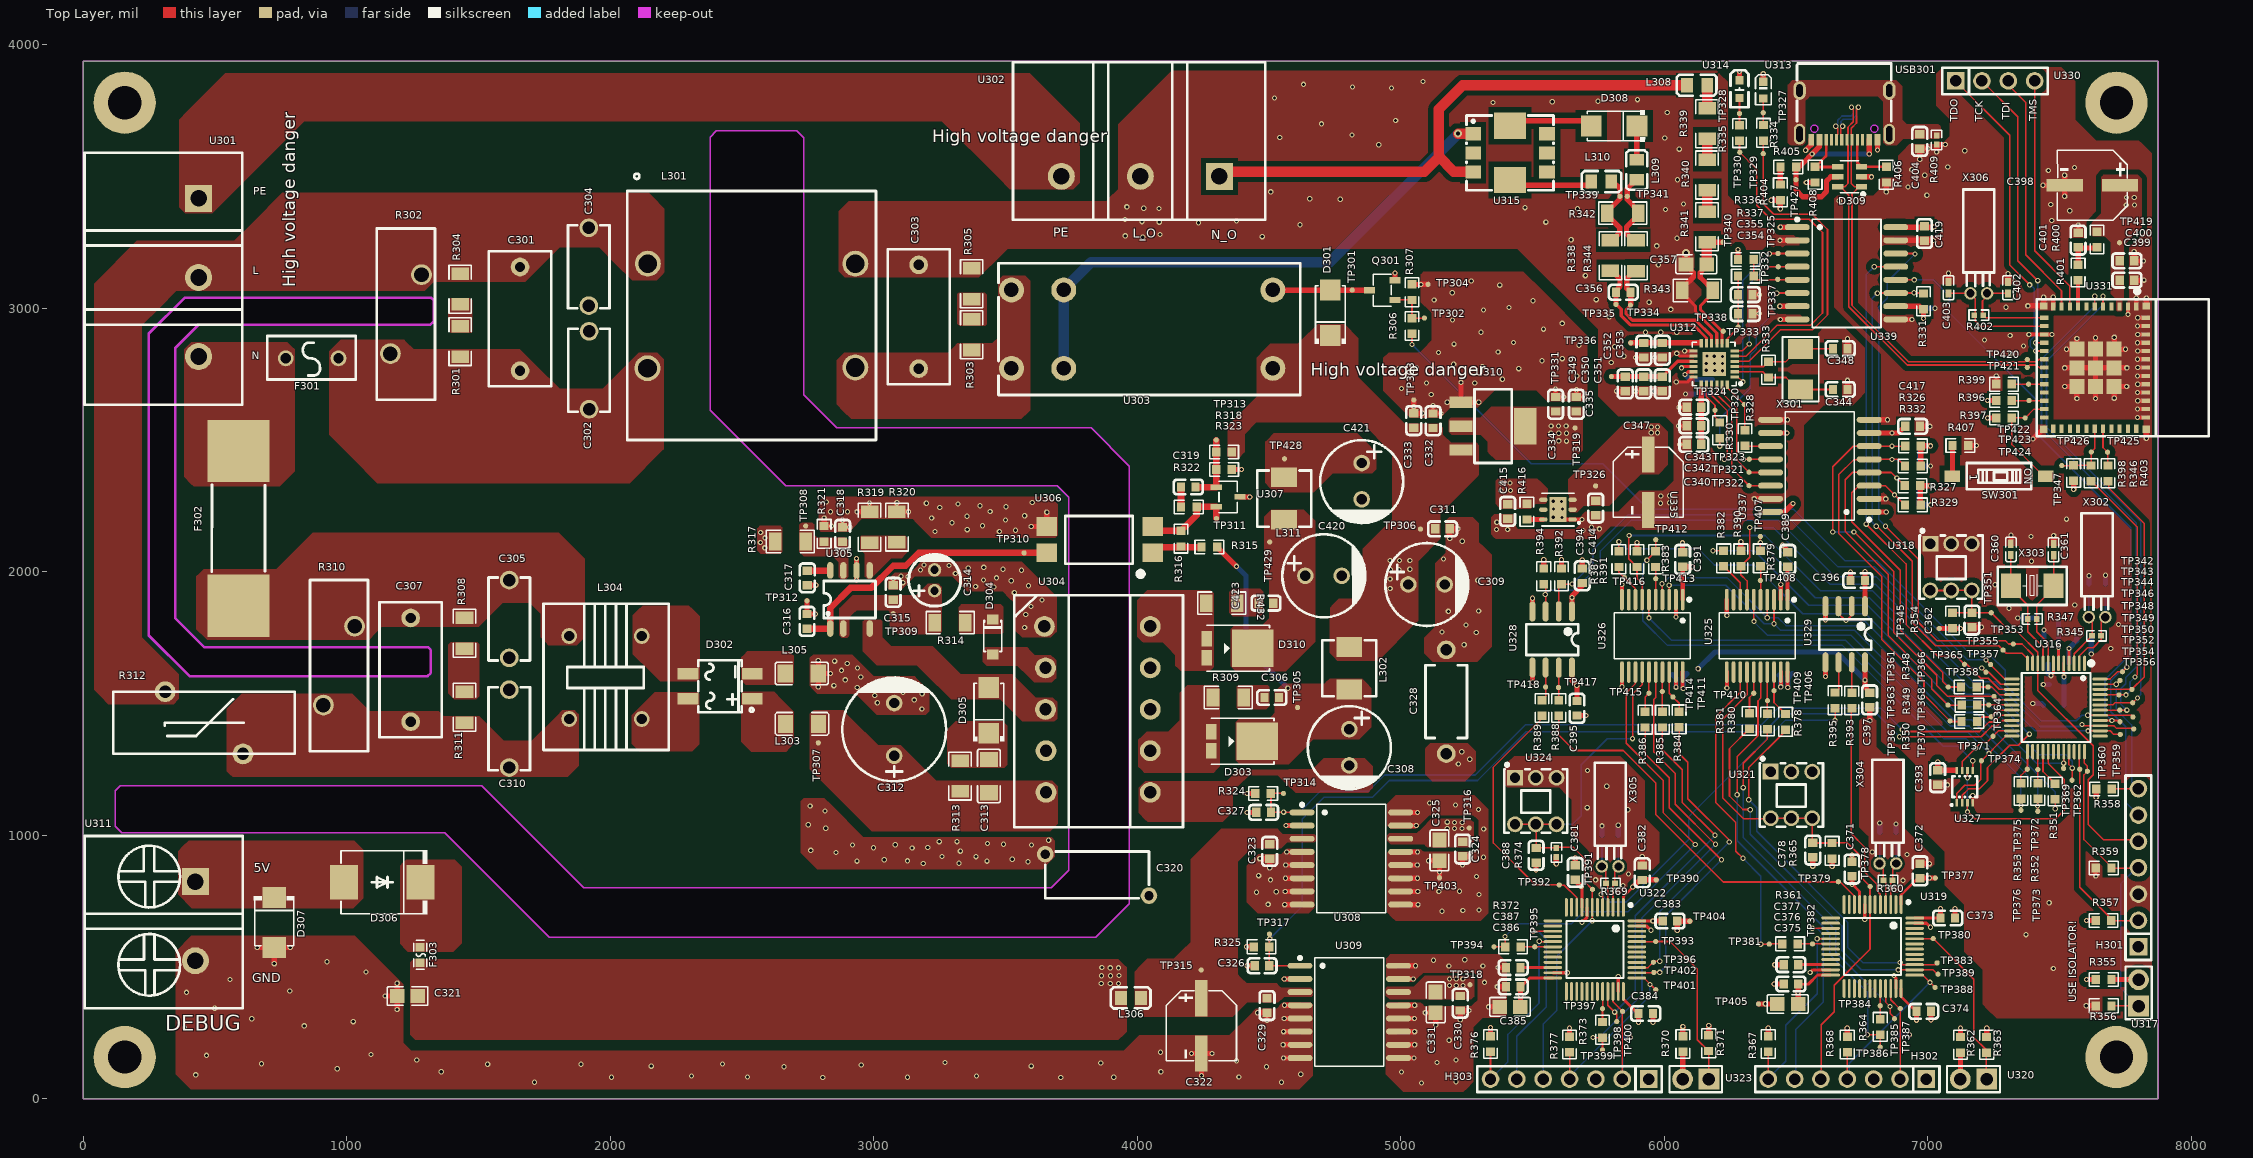
[diagram p0: Top Layer view]
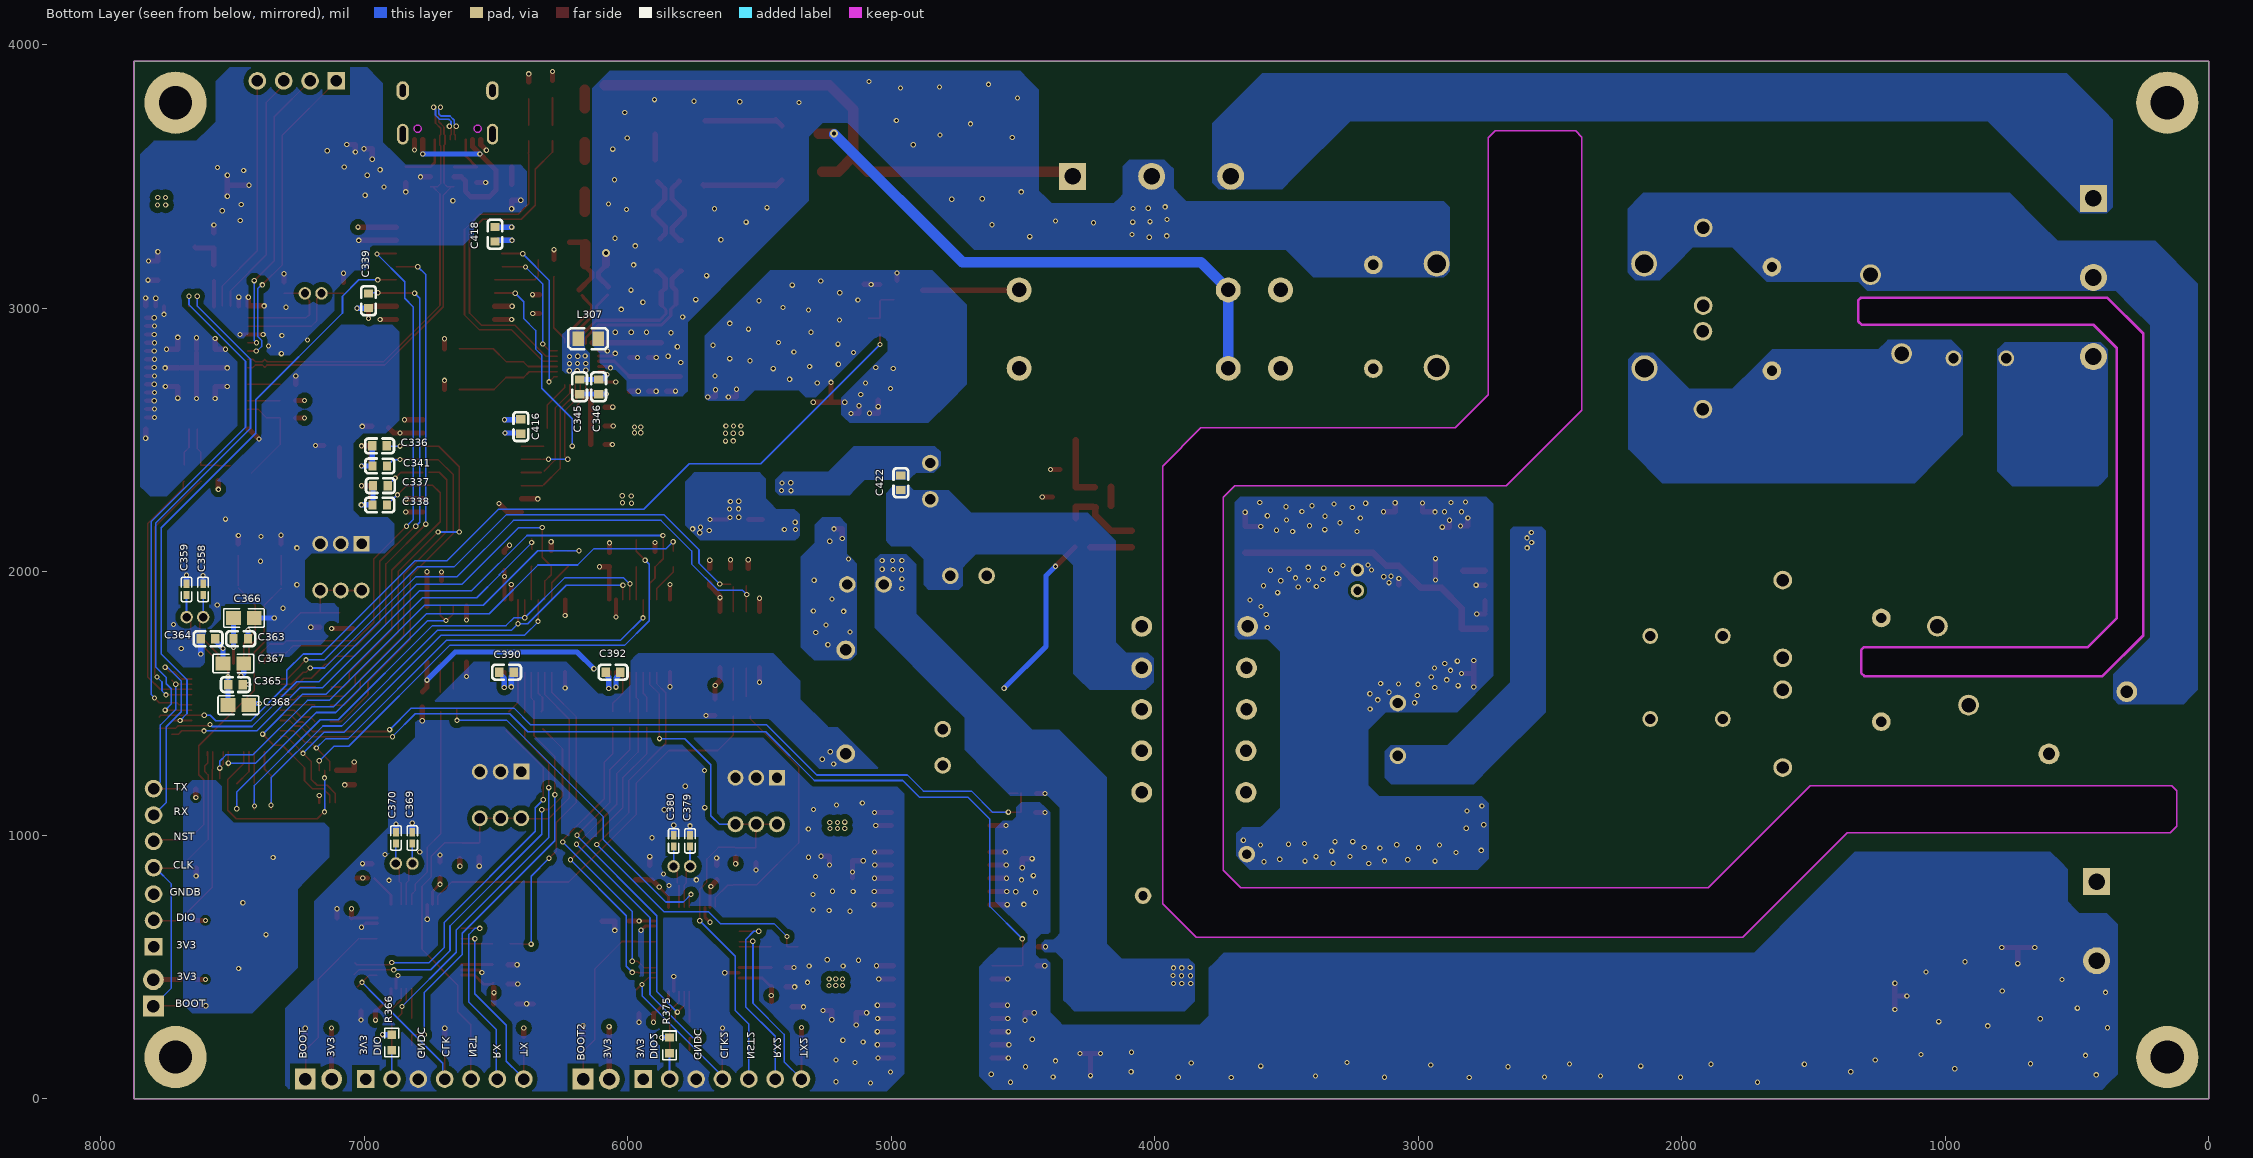
[diagram p1: Bottom Layer view, seen from below]
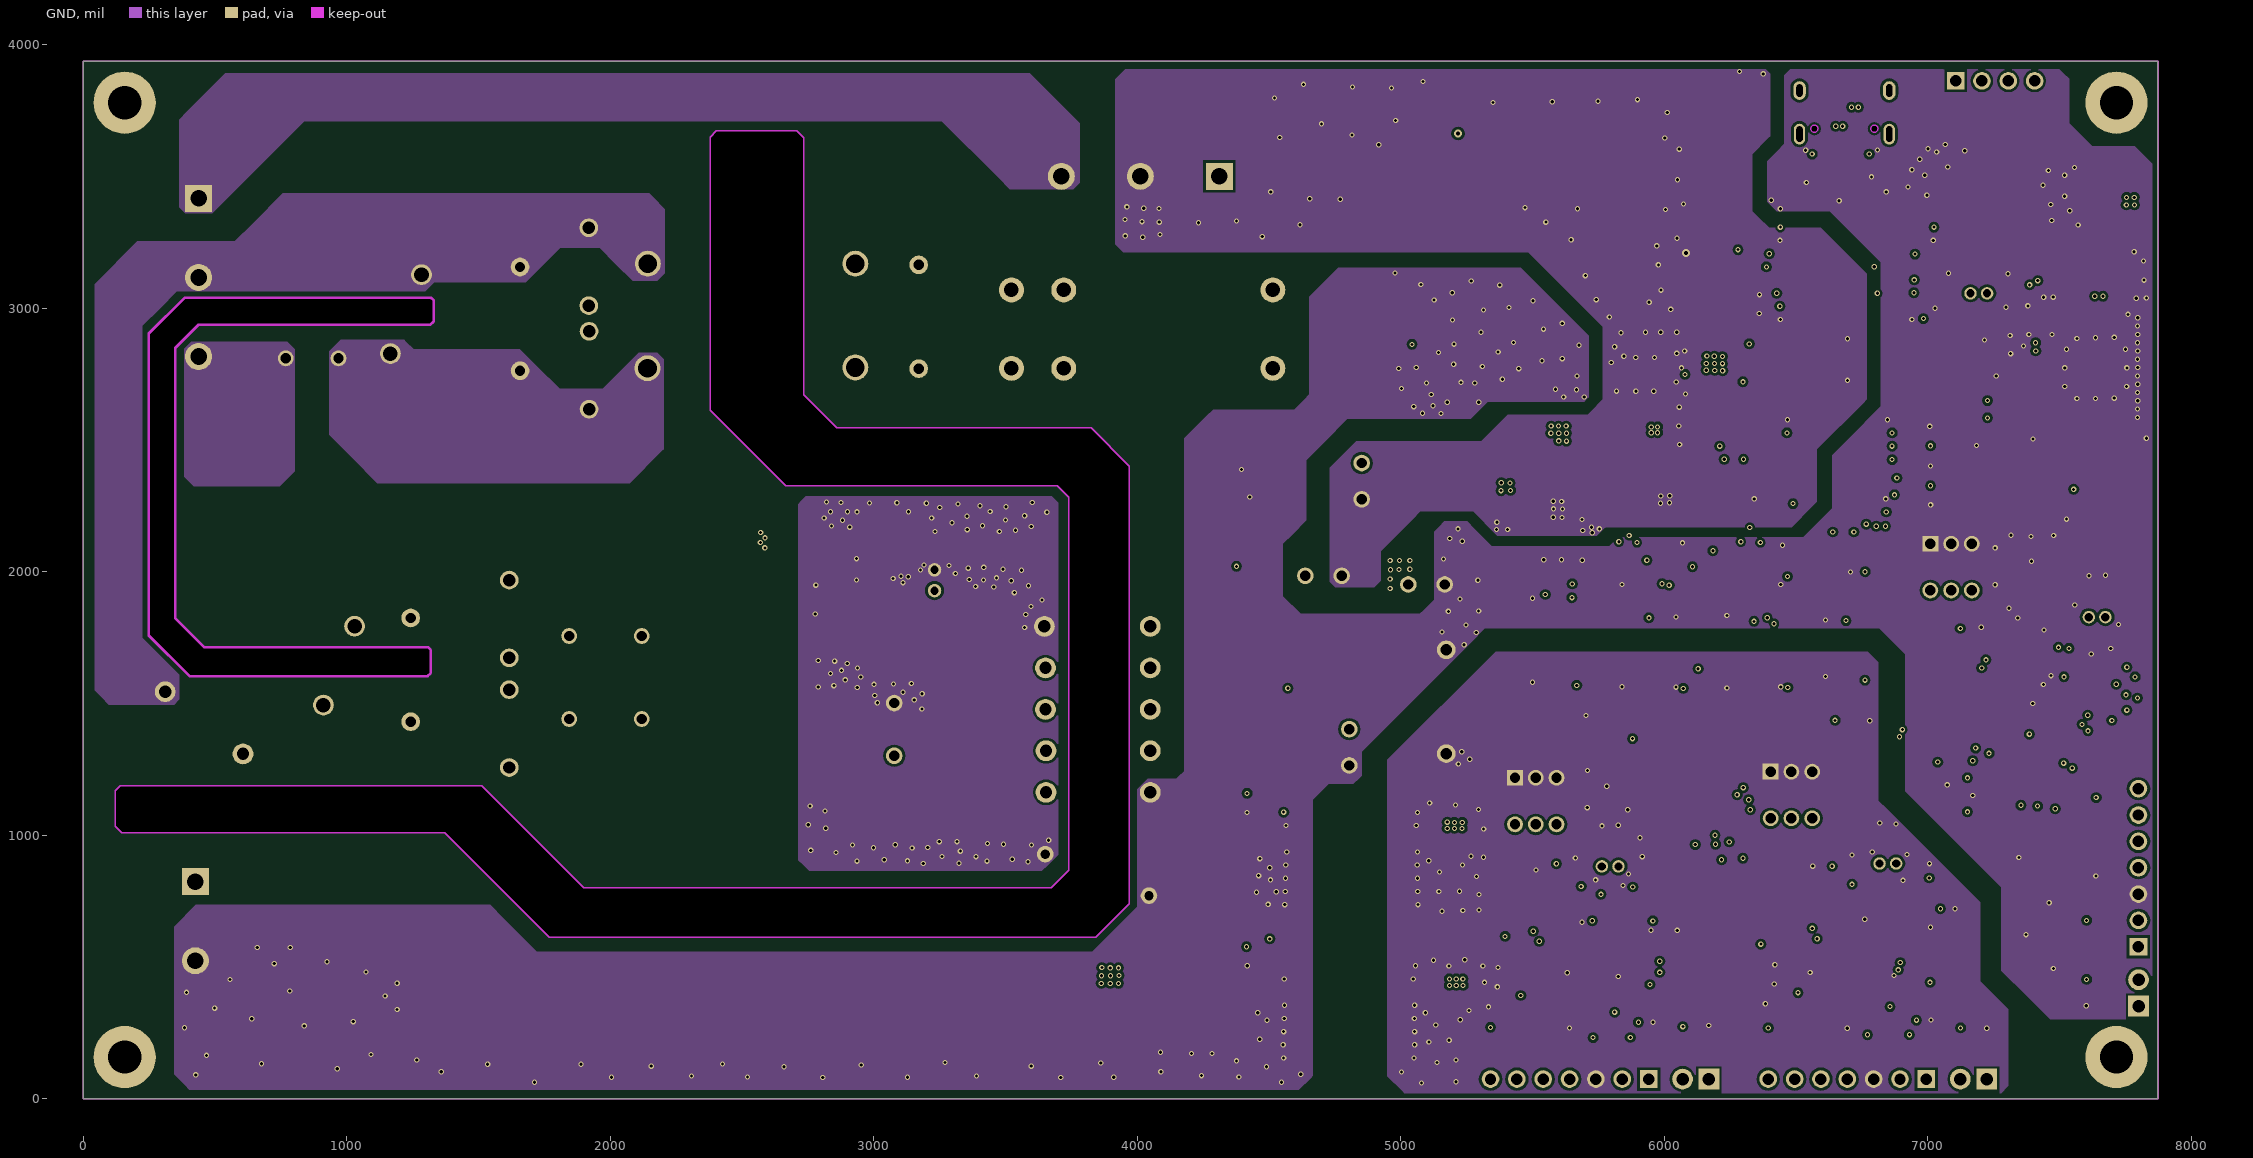
[diagram p2: GND]
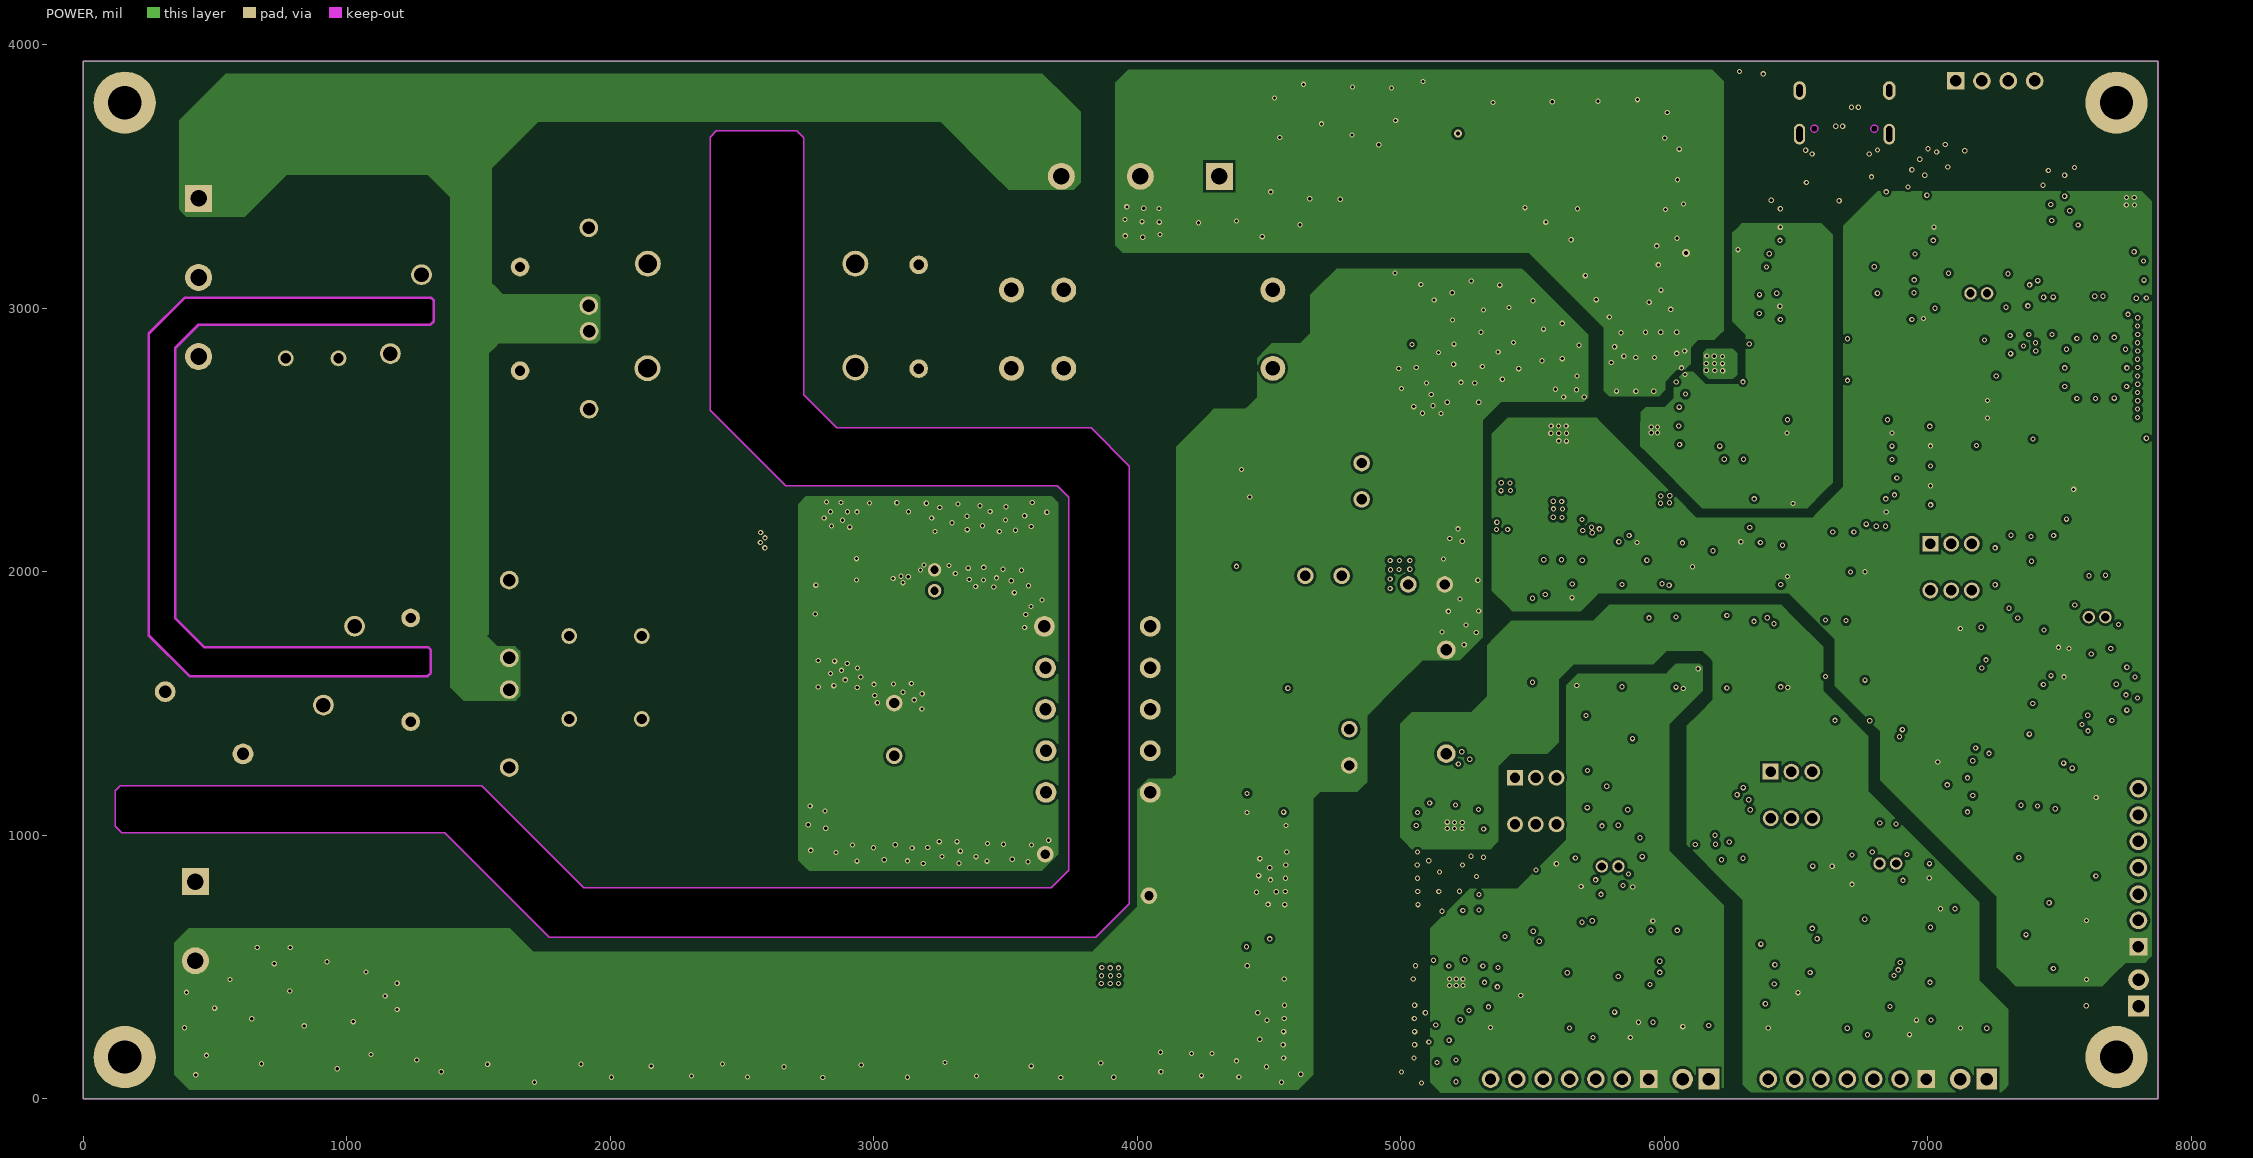
[diagram p3: POWER]
# Altium PCB MISC84429.PcbDoc (part 1 of 5)
Units mil, origin at the board's own origin, x right, y up, seen from the top; angles counter-clockwise.
Board outline 7874.02 x 3937.01 mil, 4 copper layers (Top Layer, GND, POWER, Bottom Layer); 424 components, 202 nets, 1144 pads, 784 vias.

## Layer stack, top to bottom (the 12.6 mil dielectric is the usual default, probably not edited)
Top Layer: signal copper 1.4
Dielectric: core 12.6, FR-4, Dk 4.8
GND: signal copper 1.4
Dielectric: prepreg 12.6, FR-4, Dk 4.8
POWER: signal copper 1.4
Dielectric: core 12.6, FR-4, Dk 4.8
Bottom Layer: signal copper 1.4

## Board outline
0,0 7874.02,0 7874.02,3937.01 0,3937.01
cut-out: 1769,612 1372,1009 146,1009 121,1034 121,1168 140,1187 1513,1187 1900,800 3674,800 3740,866 3740,2282 3696,2326 2666,2326 2379,2613 2379,3649 2402,3672 2709,3672 2734,3647 2734,2671 2860,2545 3825,2545 3970,2400 3970,739 3843,612
cut-out: 403.22,1602.22 248.22,1757.22 cw(c250,1759) 247.49,1759 247.49,2902 cw(c250,2902) 248.22,2903.78 384.22,3039.78 cw(c386,3038) 386,3040.51 1320,3040.51 cw(c1320,3038) 1321.78,3039.78 1329.78,3031.78 cw(c1328,3030) 1330.51,3030 1330.51,2949 cw(c1328,2949) 1329.78,2947.22 1318.78,2936.22 cw(c1317,2938) 1317,2935.49 438.04,2935.49 350.51,2847.96 350.51,1823.04 460.04,1713.51 1309,1713.51 cw(c1309,1711) 1310.78,1712.78 1318.78,1704.78 cw(c1317,1703) 1319.51,1703 1319.51,1615 cw(c1317,1615) 1318.78,1613.22 1307.78,1602.22 cw(c1306,1604) 1306,1601.49 405,1601.49 cw(c405,1604)

## Design rules (kind name [scope] priority, off if disabled: settings)
Clearance Clearance_1 [inpolygon] p1: gap=10
Clearance [All] p2: gap=6
DiffPairsRouting [All] p1: maxlimit=6 minlimit=6 mostfreqgap=6 maxuncoupledlength=500
HoleSize [All] p1: absolutevalues=TRUE maxlimit=500 minlimit=1 maxpercent=80.000 minpercent=20.000
HoleToHoleClearance [All] p1: gap=0 allowstackedmicrovias=TRUE
MinimumSolderMaskSliver [All] p1: minsoldermaskwidth=0
PlaneClearance [All] p1: clearance=6
PlaneConnect [All] p1: planeconnectstyle=Direct reliefexpansion=20 reliefentries=4 reliefconductorwidth=10 reliefairgap=10
PolygonConnect [All] p1: connectstyle=Direct reliefconductorwidth=10 reliefentries=4 polygonreliefangle="90 Angle"
RoutingVias [All] p1: holewidth=12 width=20 viastyle="Through Hole" minholewidth=12 minwidth=20 maxholewidth=12 maxwidth=20
SilkToSilkClearance [All] p1: silktosilkclearance=0
SilkscreenOverComponentPads [All] p1: minsilkscreentomaskgap=0
SolderMaskExpansion [All] p1: expansion=4
Width [All] p1: maxlimit=100 minlimit=6 preferedwidth=6
20 further rules are at their usual default settings.

## Classes and differential pairs
component class 2_2_P2_POWER: C301 C302 C303 C304 C305 C306 C307 C308 C309 C310 C311 C312 C313 C314 C315 C316 C317 C318 C319 C320 C420 C421 C422 C423 D301 D302 D303 D304 D305 D310 F301 F302 L301 L302 L303 L304 L305 L311 Q301 R301 R302 R303 R304 R305 R306 R307 R308 R309 R310 R311 R312 R313 R314 R315 R316 R317 R318 R319 R320 R321 R322 R323 R432 TP301 TP302 TP303 TP304 TP305 TP306 TP307 TP308 TP309 TP310 TP311 TP312 TP313 TP428 TP429 U301 U302 U303 U304 U305 U306 U307
component class 3_3_P3_LDO_DCDC: C321 C322 C323 C324 C325 C326 C327 C328 C329 C330 C331 C332 C333 C334 C335 D306 D307 F303 L306 R324 R325 TP314 TP315 TP316 TP317 TP318 TP319 U308 U309 U310 U311
component class 4_4_P4_STPM32: C336 C337 C338 C339 C340 C341 C342 C343 C344 C345 C346 C347 C348 C349 C350 C351 C352 C353 C354 C355 C356 C357 C414 C415 C416 C417 C418 C419 D308 L307 L308 L309 L310 R326 R327 R328 R329 R330 R331 R332 R333 R334 R335 R336 R337 R338 R339 R340 R341 R342 R343 R344 R416 TP320 TP321 TP322 TP323 TP324 TP325 TP326 TP327 TP328 TP329 TP330 TP331 TP332 TP333 TP334 TP335 TP336 TP337 TP338 TP339 TP340 TP341 U312 U313 U314 U315 U335 U337 U339 X301
component class 5_5_P5_MCU: C358 C359 C360 C361 C362 C363 C364 C365 C366 C367 C368 H301 R345 R346 R347 R348 R349 R350 R351 R352 R353 R354 R355 R356 R357 R358 R359 TP342 TP343 TP344 TP345 TP346 TP347 TP348 TP349 TP350 TP351 TP352 TP353 TP354 TP355 TP356 TP357 TP358 TP359 TP360 TP361 TP362 TP363 TP364 TP365 TP366 TP367 TP368 TP369 TP370 TP371 TP372 TP373 TP374 TP375 TP376 U316 U317 U318 X302 X303
component class 6_6_P6_AI: C369 C370 C371 C372 C373 C374 C375 C376 C377 C378 H302 R360 R361 R362 R363 R364 R365 R366 R367 R368 TP377 TP378 TP379 TP380 TP381 TP382 TP383 TP384 TP385 TP386 TP387 TP388 TP389 U319 U320 U321 X304
component class 7_7_P7_AI2: C379 C380 C381 C382 C383 C384 C385 C386 C387 C388 H303 R369 R370 R371 R372 R373 R374 R375 R376 R377 TP390 TP391 TP392 TP393 TP394 TP395 TP396 TP397 TP398 TP399 TP400 TP401 TP402 TP403 TP404 TP405 U322 U323 U324 X305
component class "9_8_P8_Translate_Tri-state gate": C389 C390 C391 C392 C393 C394 C395 C396 C397 R378 R379 R380 R381 R382 R383 R384 R385 R386 R387 R388 R389 R390 R391 R392 R393 R394 R395 TP406 TP407 TP408 TP409 TP410 TP411 TP412 TP413 TP414 TP415 TP416 TP417 TP418 U325 U326 U327 U328 U329
component class 8_9_P9_ZIGBEE: C398 C399 C400 C401 C402 C403 C404 D309 R396 R397 R398 R399 R400 R401 R402 R403 R404 R405 R406 R407 R408 R409 SW301 TP419 TP420 TP421 TP422 TP423 TP424 TP425 TP426 TP427 U330 U331 USB301 X306

## Components (designator, comment, footprint, x,y, rotation, side; value= is the part's Value field where it differs from the comment)
C301 "100nF" CAP-TH_L13.0-W6.0-P10.00-D0.6 1658,2959 r270 top
C302 "2.2nF" CAP-TH_L8.0-W4.0-P7.50-D1.2 1920,2764 r270 top
C303 "100nF" CAP-TH_L13.0-W6.0-P10.00-D0.6 3171,2967 r270 top
C304 "2.2nF" CAP-TH_L8.0-W4.0-P7.50-D1.2 1919,3157 r270 top
C305 "2.2nF" CAP-TH_L8.0-W4.0-P7.50-D1.2 1617,1820 r90 top
C306 "1nF" C0603 4511,1522 r180 top
C307 "100nF" CAP-TH_L13.0-W6.0-P10.00-D0.6 1243,1627 r90 top
C308 "680uF" CAP-TH_BD8.0-P3.50-D0.6-FD 4805,1333 r270 top
C309 "680uF" CAP-TH_BD8.0-P3.50-D0.6-FD 5098,1951 r0 top
C310 "2.2nF" CAP-TH_L8.0-W4.0-P7.50-D1.2 1617,1404 r90 top
C311 "1nF" C0603 5159,2162 r180 top
C312 "33uF" CAP-TH_BD10.0-P5.00-D1.0-FD 3078,1401 r90 top
C313 "2.2nF" C1206 3437,1224 r270 top
C314 "47uF" CAP-TH_BD5.0-P2.00-D0.8-FD 3231,1967 r90 top
C315 "100nF" C0603 3074,1921 r90 top
C316 "1nF" C0603 2747,1811 r270 top
C317 "47nF" C0603 2748,1976 r90 top
C318 "1nF" C0603 2882,2141 r270 top
C319 "100nF" C0603 4194,2321 r0 top
C320 "2.2nF" CAP-TH_L10.0-W4.5-P10.00-D0.6-S4.0 3848,849 r0 top
C321 "10uF" C0805 1231,389 r0 top
C322 "100uF" CAP-SMD_BD6.3-L6.6-W6.6-LS7.2-FD 4244,276 r270 top
C323 "22uF" C0603 4503,938 r90 top
C324 "100nF" C0603 5235,947 r270 top
C325 "10uF" C0805 5147,942 r90 top
C326 "1uF" C0603 4474,504 r0 top
C327 "1uF" C0603 4480,1086 r0 top
C328 "100pF" CAP-TH_L7.0-W4.0-P10.00-D0.6 5173,1506 r270 top
C329 "22uF" C0603 4493,353 r90 top
C330 "100nF" C0603 5226,362 r270 top
C331 "10uF" C0805 5133,365 r90 top
C332 "2.2uF" C0603 5123,2572 r270 top
C333 "100nF" C0603 5049.82,2573.19 r90 top
C334 "4.7uF" C0603 5588,2635 r270 top
C335 "100nF" C0603 5667,2635 r90 top
C336 "150pF" C0603 6942.21,2476.86 r0 bottom
C337 "150pF" C0603 6939.21,2325.86 r0 bottom
C338 "150pF" C0603 6941.21,2252.86 r0 bottom
C339 "150pF" C0603 6984,3028 r270 bottom
C340 "100nF" C0603 6112.98,2482.54 r180 top
C341 "150pF" C0603 6941.21,2400.86 r0 bottom
C342 "150pF" C0603 6112.98,2552.79 r180 top
C343 "4.7uF" C0603 6113,2624 r0 top
C344 "15pF" C0603 6668,2691 r180 top
C345 "150pF" C0603 6183,2701 r270 bottom
C346 "100nF" C0603 6111,2701 r270 bottom
C347 "100uF" CAP-SMD_BD6.3-L6.6-W6.6-LS7.3-FD-H7.7 5939,2339 r270 top
C348 "15pF" C0603 6668,2846 r180 top
C349 "150pF" C0603 5852.28,2712.26 r90 top
C350 "100nF" C0603 5922,2712 r90 top
C351 "1uF" C0603 5993,2712 r90 top
C352 "150pF" C0603 5923,2840 r90 top
C353 "100nF" C0603 5993,2840 r90 top
C354 "150pF" C0603 6308,2979 r180 top
C355 "100nF" C0603 6308,3051 r180 top
C356 "10nF" C0603 5845,3060 r180 top
C357 "22nF" C0805 6122,3166 r0 top
C358 "15pF" C0402 7612,1932 r270 bottom
C359 "15pF" C0402 7675,1932 r90 bottom
C360 "30pF" C0402 7316,2084 r90 top
C361 "30pF" C0402 7478,2083 r270 top
C362 "1uF" C0603 7168,1816 r90 top
C363 "100nF" C0603 7469,1745 r180 bottom
C364 "100nF" C0603 7593,1745 r0 bottom
C365 "100nF" C0603 7489,1571 r180 bottom
C366 "10uF" C0805 7457,1824 r0 bottom
C367 "10uF" C0805 7497,1651 r0 bottom
C368 "10uF" C0805 7478,1493 r0 bottom
C369 "15pF" C0402 6818,989 r270 bottom
C370 "15pF" C0402 6880,989 r90 bottom
C371 "100nF" C0603 6713,871 r90 top
C372 "100nF" C0603 6971,864 r90 top
C373 "100nF" C0603 7076,685 r0 top
C374 "100nF" C0603 6985,331 r0 top
C375 "10uF" C0805 6469,359 r0 top
C376 "1nF" C0603 6481,435 r0 top
C377 "4.7uF" C0603 6481,508 r180 top
C378 "1uF" C0603 6564,943 r90 top
C379 "15pF" C0402 5764,978 r270 bottom
C380 "15pF" C0402 5826,978 r90 bottom
C381 "100nF" C0603 5663,858 r90 top
C382 "100nF" C0603 5917,857 r90 top
C383 "100nF" C0603 6022,674 r0 top
C384 "100nF" C0603 5930,323 r0 top
C385 "10uF" C0805 5415,348 r0 top
C386 "1nF" C0603 5427,424 r0 top
C387 "4.7uF" C0603 5427,497 r180 top
C388 "1uF" C0603 5514,923 r90 top
C389 "100nF" C0603 6469,2046 r90 top
C390 "100nF" C0603 6460,1618 r180 bottom
C391 "100nF" C0603 6070,2046 r90 top
C392 "100nF" C0603 6056,1618 r180 bottom
C393 "100nF" C0603 7038,1218 r270 top
C394 "100nF" C0603 5689,1984 r90 top
C395 "100nF" C0603 5669,1481 r270 top
C396 "100nF" C0603 6735,1966 r180 top
C397 "100nF" C0603 6780,1513 r270 top
C398 "100uF" CAP-SMD_BD6.3-L6.6-W6.6-LS7.2-FD 7625,3466 r180 top
C399 "100nF" C0603 7756,3106 r180 top
C400 "22uF" C0603 7756,3179 r0 top
C401 "1uF" C0603 7571,3258 r270 top
C402 "15pF" C0402 7305,3077 r270 top
C403 "15pF" C0402 7079,3077 r90 top
C404 "10nF" C0603 6970,3632.44 r90 top
C414 "4.7uF" C0603 5740,2241 r90 top
C415 "1uF" C0603 5406,2228 r90 top
C416 "100nF" C0603 6406,2550 r90 bottom
C417 "100nF" C0603 6943,2551 r0 top
C418 "100nF" C0603 6504,3280 r270 bottom
C419 "100nF" C0603 6988,3283 r270 top
C420 "680uF" CAP-TH_BD8.0-P3.50-D0.6-FD 4707,1984 r0 top
C421 "680uF" CAP-TH_BD8.0-P3.50-D0.6-FD 4852,2343 r270 top
C422 "1nF" C0603 4964,2337 r90 bottom
C423 "1nF" C0603 4489,1880 r180 top
D301 "SS14" SMA_L4.3-W2.6-LS5.2-RD 4733,2982 r90 top
D302 "MB10S-50MIL" MBS_L4.7-W3.8-P2.40-LS7.0-TL 2417,1565 r180 top
D303 "SB10100L" TO-277A_L4.7-W6.1-LS6.6-TR 4368,1356 r180 top
D304 "BAV21W" SOD-123_L2.8-W1.8-LS3.7-RD 3452,1752 r270 top
D305 "FR107(RS1M)" SMA_L4.3-W2.6-LS5.2-RD 3437,1473 r90 top
D306 "SS34" SMC_L6.9-W5.9-LS7.9-RD 1135,821 r180 top
D307 "SMBJ5.0A" SMB_L4.6-W3.6-LS5.4-RD 725,668 r270 top
D308 "SS14" SMA_L4.3-W2.6-LS5.2-RD 5810,3691 r180 top
D309 "SRV05-4" SOT-23-6_L2.9-W1.6-P0.95-LS2.8-BL 6704,3498 r90 top
D310 "SB10100L" TO-277A_L4.7-W6.1-LS6.6-TR 4351,1709 r180 top
F301 "20A250VVS" FUSE-TH_L8.4-W4.0-P5.08-D0.6 869,2809 r0 top
F302 "SGT520-2A T2AL250V" FUSE-SMD_L20.0-W5.0 590,2164 r270 top
F303 "SMD0603-010-15" F0603 1279,545 r90 top
H301 "PZ254V-11-07P" HDR-TH_7P-P2.54-V-M 7799.94,876.06 r90 top
H302 "PZ254V-11-07P" HDR-TH_7P-P2.54-V-M 6695,74 r180 top
H303 "PZ254V-11-07P" HDR-TH_7P-P2.54-V-M 5641,74 r180 top
L301 "FC-DLFW2015-5mH-20A-LF" FILTER-TH_FC-DLFW2015-5MH-20A-LF 2536,2970 r270 top
L302 "4.7uH" IND-SMD_L5.4-W5.2_FXL0530 4805,1633 r90 top
L303 "" L1206 2728,1422 r0 top
L304 "DLSF1010-12mH-L-S" IND-TH_4P-L14.0-W12.0_DLSF1010-12MH-L-S 1982,1598 r270 top
L305 "" L1206 2727,1613 r0 top
L306 "BLM21PG221SN1D" L0805 3977,382 r0 top
L307 "" L0805 6150,2884 r180 bottom
L308 "" L0805 6125,3846 r0 top
L309 "" L0805 5896,3525 r90 top
L310 "" L0805 5761,3480 r180 top
L311 "4.7uH" IND-SMD_L5.4-W5.2_FXL0530 4558,2277 r90 top
Q301 "MMBT3904LT1G" SOT-23-3_L2.9-W1.6-P1.90-LS2.8-BR 4930,3068 r0 top
R301 "" R1206 1431,2873 r270 top
R302 "430pF@1kHz" RES-TH_L16.5-W5.6-P7.50-D1.2-S3.00 1225,2977 r270 top
R303 "" R1206 3372,2899 r270 top
R304 "" R1206 1431,3072 r270 top
R305 "" R1206 3372,3092 r270 top
R306 "" R0603 5043,2932 r90 top
R307 "" R0603 5043,3060 r90 top
R308 "" R1206 1447,1766 r90 top
R309 "" R1206 4346,1522 r0 top
R310 "430pF@1kHz" RES-TH_L16.5-W5.6-P7.50-D1.2-S3.00 971,1643 r90 top
R311 "" R1206 1447,1485 r90 top
R312 "MF72 20D15" RES-TH_L17.5-W6.0-P7.50-D0.8-S7.50 459,1426 r0 top
R313 "" R1206 3328,1224 r270 top
R314 "" R1206 3290,1806 r0 top
R315 "" R0603 4274,2093 r0 top
R316 "" R0603 4166,2125 r270 top
R317 "" R1206 2684,2114 r0 top
R318 "" R0603 4330,2454 r0 top
R319 "" R1206 2984.62,2168.34 r270 top
R320 "" R1206 3088,2169 r270 top
R321 "" R0603 2812,2143 r270 top
R322 "" R0603 4196,2245 r180 top
R323 "" R0603 4330,2387 r180 top
R324 "" R0603 4478,1158 r180 top
R325 "" R0603 4472,576 r180 top
R326 "" R0603 6944.66,2477.1 r180 top
R327 "" R0603 6942.66,2325.75 r180 top
R328 "" R0603 6307,2507 r270 top
R329 "" R0603 6943.66,2253.1 r180 top
R330 "" R0603 6211,2536 r270 top
R331 "" R0603 6983.89,3025.55 r90 top
R332 "" R0603 6943.66,2401 r180 top
R333 "" R0603 6396,2766 r270 top
R334 "" R0603 6376.74,3664.98 r270 top
R335 "" R0603 6286,3664 r270 top
R336 "" R0603 6310,3184 r180 top
R337 "" R0603 6310,3121 r0 top
R338 "" R1206 5796,3199 r90 top
R339 "" R1206 6163,3700 r90 top
R340 "" R1206 6163,3505 r270 top
R341 "" R1206 6163,3308 r90 top
R342 "" R1206 5843,3360 r180 top
R343 "" R1206 6126,3067 r0 top
R344 "" R1206 5893.1,3198.77 r90 top
R345 "" R0402 7641,1756 r180 top
R346 "" R0603 7620,2373 r270 top
R347 "" R0402 7397,1820 r180 top
R348 "" R0603 7156,1562 r180 top
R349 "" R0603 7159,1493 r180 top
R350 "" R0603 7158,1431 r180 top
R351 "" R0603 7484,1165 r90 top
R352 "" R0603 7418,1167 r90 top
R353 "" R0603 7354,1167 r90 top
R354 "" R0603 7094,1814 r270 top
R355 "" R0603 7668,452 r180 top
R356 "" R0603 7668,352 r180 top
R357 "" R0603 7667,676 r180 top
R358 "" R0603 7669,1175 r180 top
R359 "" R0603 7668,875 r180 top
R360 "" R0402 6850,828 r180 top
R361 "" R0603 6478,587 r180 top
R362 "" R0603 7125,204 r90 top
R363 "" R0603 7224,204 r90 top
R364 "" R0603 6820,272 r90 top
R365 "" R0603 6637.57,940.13 r270 top
R366 "" R0603 6896,213 r90 bottom
R367 "" R0603 6395,207 r90 top
R368 "" R0603 6695,205 r90 top
R369 "" R0402 5796,817 r180 top
R370 "" R0603 6071,207 r90 top
R371 "" R0603 6169,210 r270 top
R372 "" R0603 5426,576 r180 top
R373 "" R0603 5766,261 r90 top
R374 "" R0402 5590.95,933.48 r270 top
R375 "" R0603 5842,202 r90 bottom
R376 "" R0603 5341,207 r90 top
R377 "" R0603 5641,205 r90 top
R378 "" R0603 6461,1430 r90 top
R379 "" R0603 6365,2050 r90 top
R380 "" R0603 6392,1431 r90 top
R381 "" R0603 6323,1433 r90 top
R382 "" R0603 6226,2050 r90 top
R383 "" R0603 5968,2047 r90 top
R384 "" R0603 6057,1439 r90 top
R385 "" R0603 5993,1438 r90 top
R386 "" R0603 5928,1438 r90 top
R387 "" R0603 5828,2047 r90 top
R388 "" R0603 5600,1482 r90 top
R389 "" R0603 5536,1482 r90 top
R390 "" R0603 6291,2050 r270 top
R391 "" R0603 5897,2047 r270 top
R392 "" R0603 5610,1982 r90 top
R393 "" R0603 6712,1511 r90 top
R394 "" R0603 5543,1982 r90 top
R395 "" R0603 6648.74,1511.12 r90 top
R396 "" R0603 7290,2649 r180 top
R397 "" R0603 7290,2583 r180 top
R398 "" R0603 7554,2374 r270 top
R399 "" R0603 7290,2711 r0 top
R400 "" R0603 7643,3260 r90 top
R401 "" R0603 7571,3135 r270 top
R402 "" R0402 7194,2973 r0 top
R403 "" R0603 7684,2373 r90 top
R404 "" R0603 6441,3439 r270 top
R405 "" R0603 6471,3535 r0 top
R406 "" R0603 6843,3506 r90 top
R407 "" R0603 7124,2478 r180 top
R408 "" R0603 6573,3506 r90 top
R409 "" R0402 7034,3638 r90 top
R416 "" R0603 5479,2227 r270 top
R432 "" R1206 4321,1880 r0 top
SW301 "U903" SW-SMD_2P-L3.5-W6.1-P2.54-LS9.8 7271,2362 r0 top
TP301 "" Test-Point-0.5mm 4816,3068 r180 top
TP302 "" Test-Point-0.5mm 5090,2962 r90 top
TP303 "" Test-Point-0.5mm 5050,2651 r90 top
TP304 "" Test-Point-0.5mm 5104,3090 r90 top
TP305 "" Test-Point-0.5mm 4609,1484 r0 top
TP306 "" Test-Point-0.5mm 5075,2161 r180 top
TP307 "" Test-Point-0.5mm 2790,1350 r0 top
TP308 "" Test-Point-0.5mm 2742,2173 r0 top
TP309 "" Test-Point-0.5mm 3074,1840 r0 top
TP310 "" Test-Point-0.5mm 3571,2071 r0 top
TP311 "" Test-Point-0.5mm 4301,2201 r0 top
TP312 "" Test-Point-0.5mm 2747,1889 r0 top
TP313 "" Test-Point-0.5mm 4300,2499 r0 top
TP314 "" Test-Point-0.5mm 4555,1158 r0 top
TP315 "" Test-Point-0.5mm 4243,488 r180 top
TP316 "" Test-Point-0.5mm 5260,1027 r0 top
TP317 "" Test-Point-0.5mm 4502,624 r0 top
TP318 "" Test-Point-0.5mm 5263,432 r0 top
TP319 "" Test-Point-0.5mm 5662,2545 r0 top
TP320 "" Test-Point-0.5mm 6304,2634 r180 top
TP321 "" Test-Point-0.5mm 6322,2377 r270 top
TP322 "" Test-Point-0.5mm 6322,2326 r270 top
TP323 "" Test-Point-0.5mm 6323,2426 r270 top
TP324 "" Test-Point-0.5mm 6193,2612 r180 top
TP325 "" Test-Point-0.5mm 6432,3207 r0 top
TP326 "" Test-Point-0.5mm 5740,2325 r180 top
TP327 "" Test-Point-0.5mm 6376,3741 r180 top
TP328 "" Test-Point-0.5mm 6286,3738 r180 top
TP329 "" Test-Point-0.5mm 6376,3586 r180 top
TP330 "" Test-Point-0.5mm 6287,3591 r180 top
TP331 "" Test-Point-0.5mm 5800,2740 r90 top
TP332 "" Test-Point-0.5mm 6433,3157 r0 top
TP333 "" Test-Point-0.5mm 6224,2912 r90 top
TP334 "" Test-Point-0.5mm 5872,3011 r90 top
TP335 "" Test-Point-0.5mm 5817,3014 r90 top
TP336 "" Test-Point-0.5mm 5873,2868 r90 top
TP337 "" Test-Point-0.5mm 6431,3109 r90 top
TP338 "" Test-Point-0.5mm 6281,2928 r90 top
TP339 "" Test-Point-0.5mm 5832,3424 r90 top
TP340 "" Test-Point-0.5mm 6223,3250 r90 top
TP341 "" Test-Point-0.5mm 5860,3424 r90 top
TP342 "" Test-Point-0.5mm 7739,1620 r0 top
TP343 "" Test-Point-0.5mm 7730,1587 r0 top
TP344 "" Test-Point-0.5mm 7775,1553 r0 top
TP345 "" Test-Point-0.5mm 7044,1784 r180 top
TP346 "" Test-Point-0.5mm 7726,1532 r0 top
TP347 "" Test-Point-0.5mm 7509,2402 r270 top
TP348 "" Test-Point-0.5mm 7778,1502 r0 top
TP349 "" Test-Point-0.5mm 7729,1474 r0 top
TP350 "" Test-Point-0.5mm 7779,1448 r0 top
TP351 "" Test-Point-0.5mm 7241.44,1843.56 r180 top
TP352 "" Test-Point-0.5mm 7730,1430 r0 top
TP353 "" Test-Point-0.5mm 7325,1725 r180 top
TP354 "" Test-Point-0.5mm 7782,1403 r0 top
TP355 "" Test-Point-0.5mm 7286,1702 r180 top
TP356 "" Test-Point-0.5mm 7731,1382 r0 top
TP357 "" Test-Point-0.5mm 7239,1647 r180 top
TP358 "" Test-Point-0.5mm 7221,1618 r180 top
TP359 "" Test-Point-0.5mm 7606,1242 r0 top
TP360 "" Test-Point-0.5mm 7577,1250 r0 top
TP361 "" Test-Point-0.5mm 7078,1562 r180 top
TP362 "" Test-Point-0.5mm 7548,1208 r270 top
TP363 "" Test-Point-0.5mm 7077,1493 r180 top
TP364 "" Test-Point-0.5mm 7252,1526 r180 top
TP365 "" Test-Point-0.5mm 7140,1648 r180 top
TP366 "" Test-Point-0.5mm 7229,1562 r180 top
TP367 "" Test-Point-0.5mm 7085,1433 r180 top
TP368 "" Test-Point-0.5mm 7232,1494 r180 top
TP369 "" Test-Point-0.5mm 7516,1253 r270 top
TP370 "" Test-Point-0.5mm 7241,1449 r180 top
TP371 "" Test-Point-0.5mm 7248,1375 r180 top
TP372 "" Test-Point-0.5mm 7418,1249 r270 top
TP373 "" Test-Point-0.5mm 7418,1090 r180 top
TP374 "" Test-Point-0.5mm 7204,1282 r180 top
TP375 "" Test-Point-0.5mm 7378,1250 r270 top
TP376 "" Test-Point-0.5mm 7354,1094 r180 top
TP377 "" Test-Point-0.5mm 7029,837 r180 top
TP378 "" Test-Point-0.5mm 6782,805 r180 top
TP379 "" Test-Point-0.5mm 6661,823 r180 top
TP380 "" Test-Point-0.5mm 7021,607 r180 top
TP381 "" Test-Point-0.5mm 6399,586 r180 top
TP382 "" Test-Point-0.5mm 6563,587 r180 top
TP383 "" Test-Point-0.5mm 7036,515 r180 top
TP384 "" Test-Point-0.5mm 6820,352 r180 top
TP385 "" Test-Point-0.5mm 6874,303 r180 top
TP386 "" Test-Point-0.5mm 6820,195 r180 top
TP387 "" Test-Point-0.5mm 6896,342 r180 top
TP388 "" Test-Point-0.5mm 7028,422 r180 top
TP389 "" Test-Point-0.5mm 7039,472 r180 top
TP390 "" Test-Point-0.5mm 5970,830 r180 top
TP391 "" Test-Point-0.5mm 5728,794 r180 top
TP392 "" Test-Point-0.5mm 5602,811 r180 top
TP393 "" Test-Point-0.5mm 5968,596 r180 top
TP394 "" Test-Point-0.5mm 5354,576 r180 top
TP395 "" Test-Point-0.5mm 5509,576 r180 top
TP396 "" Test-Point-0.5mm 5959,517 r180 top
TP397 "" Test-Point-0.5mm 5766,341 r180 top
TP398 "" Test-Point-0.5mm 5820,292 r180 top
TP399 "" Test-Point-0.5mm 5766,184 r180 top
TP400 "" Test-Point-0.5mm 5842,331 r180 top
TP401 "" Test-Point-0.5mm 5968,413 r180 top
TP402 "" Test-Point-0.5mm 5961,479 r180 top
TP403 "" Test-Point-0.5mm 5147,838 r180 top
TP404 "" Test-Point-0.5mm 6097,673 r180 top
TP405 "" Test-Point-0.5mm 6358,359 r180 top
TP406 "" Test-Point-0.5mm 6417,1548 r270 top
TP407 "" Test-Point-0.5mm 6365,2133 r270 top
TP408 "" Test-Point-0.5mm 6365,1966 r270 top
TP409 "" Test-Point-0.5mm 6392,1510 r270 top
TP410 "" Test-Point-0.5mm 6340,1538 r270 top
TP411 "" Test-Point-0.5mm 6033,1524 r270 top
TP412 "" Test-Point-0.5mm 5968,2121 r270 top
TP413 "" Test-Point-0.5mm 5968,1973 r270 top
TP414 "" Test-Point-0.5mm 5993,1545 r270 top
TP415 "" Test-Point-0.5mm 5942,1538 r270 top
TP416 "" Test-Point-0.5mm 5848.98,1977.02 r270 top
TP417 "" Test-Point-0.5mm 5599,1560 r270 top
TP418 "" Test-Point-0.5mm 5550,1562 r270 top
TP419 "" Test-Point-0.5mm 7728,3248 r270 top
TP420 "" Test-Point-0.5mm 7378,2805 r270 top
TP421 "" Test-Point-0.5mm 7378,2775 r270 top
TP422 "" Test-Point-0.5mm 7383,2711 r270 top
TP423 "" Test-Point-0.5mm 7385,2649 r270 top
TP424 "" Test-Point-0.5mm 7370,2583 r270 top
TP425 "" Test-Point-0.5mm 7683,2453 r270 top
TP426 "" Test-Point-0.5mm 7621,2454 r270 top
TP427 "" Test-Point-0.5mm 6500,3487 r180 top
TP428 "" Test-Point-0.5mm 4559,2428 r90 top
TP429 "" Test-Point-0.5mm 4503,2112 r90 top
U301 "DBT50G-7.62-3P-BK-P" CONN-TH_3P-P7.62_L15.2-W24.4-EX4.2 438,3116 r270 top
U302 "DBT50G-7.62-3P-BK-P" CONN-TH_3P-P7.62_L15.2-W24.4-EX4.2 4012,3500 r180 top
U303 "HF115F-I/005-1HS3A" RELAY-TH_HF115F-XXX-1HS3 4019,2920 r180 top
U304 "" 111 3534,1910 r0 top
U305 "HF500GS-15-Z" SOIC-8_7P-L4.9-W3.9-P1.27-LS6.0-BL-PE3 2910,1894 r0 top
U306 "PC817AS" SOP-4_L6.5-W4.6-P2.54-LS10.2-TL 3858,2121 r180 top
U307 "TL431KB-TP" SOT-23-3_L2.9-W1.4-P1.91-LS2.6-BR 4345,2283 r180 top
U308 "CA-IS3115AW" SOIC-16_L10.3-W7.5-P1.27-LS10.3-BL 4813,911 r270 top
U309 "CA-IS3115AW" SOIC-16_L10.3-W7.5-P1.27-LS10.3-BL 4805,329 r270 top
U310 "TLV1117LV33DCYR" SOT-223_L6.7-W3.5-P2.30-BR 5351,2552 r180 top
U311 "DBT50G-7.62-2P-BK-P" CONN-TH_2P-P7.62_L15.2-W16.7-EX4.2 426,673 r270 top
U312 "STPM32TR" VQFN-24_L4.0-W4.0-P0.50-BL-EP2.3 6190,2788 r90 top locked
U313 "19-217/GHC-YR1S2/6T" LED0603-RD_GREEN 6376,3827 r270 top
U314 "19-217/R6C-AL1M2VY/6T" LED0603-R-FD 6286,3831 r270 top
U315 "PA1005.100NL" SENSOR-TH_PA1005.100NL 5415,3589 r90 top
U316 "STM32G071CBT6" LQFP-48_L7.0-W7.0-P0.50-LS9.0-BL 7487,1484 r180 top
U317 "PZ254V-11-02P" HDR-TH_2P-P2.54-V-M 7800.51,400.98 r90 top
U318 "5.8 ZSGT" SW-TH_5.8ZSGT 7089,2017 r180 top
U319 "STM32U575CGT6" LQFP-48_L7.0-W7.0-P0.50-LS9.0-TL 6791,577 r270 top
U320 "PZ254V-11-02P" HDR-TH_2P-P2.54-V-M 7173.99,73.79 r180 top
U321 "5.8 ZSGT" SW-TH_5.8ZSGT 6482.85,1152.12 r180 top
U322 "STM32U575CGT6" LQFP-48_L7.0-W7.0-P0.50-LS9.0-TL 5737,566 r270 top
U323 "PZ254V-11-02P" HDR-TH_2P-P2.54-V-M 6119.99,73.79 r180 top
U324 "5.8 ZSGT" SW-TH_5.8ZSGT 5512.85,1129.12 r180 top
U325 "ADUM3150BRSZ-RL7" SSOP-20_L7.2-W5.3-P0.65-LS7.8-BL 6353,1756 r180 top
U326 "ADUM3150BRSZ-RL7" SSOP-20_L7.2-W5.3-P0.65-LS7.8-BL 5955,1756 r180 top
U327 "SN74LVC2G125DCUR" VSON8_L2.0-W2.3-P0.50-LS3.1-BL 7141,1184 r0 top
U328 "ISO7720FDR" SOIC-8_L5.0-W4.0-P1.27-LS6.1-BL 5575,1742 r180 top
U329 "ISO7720FDR" SOIC-8_L5.0-W4.0-P1.27-LS6.1-BL 6687,1762 r180 top
U330 "PZ254V-11-04P" HDR-TH_4P-P2.54-V-M 7256,3862 r0 top
U331 "ESP32-C6-MINI-1-N4" WIFIM-SMD_61P-L16.6-W13.2-P0.80-ESP32-C6-MINI-1-N4 7635,2774 r270 top
U335 "LDL212PU33R" VSON-6_L3.0-W3.0-P0.95-TL-EP_TI_DRP 5597,2235 r180 top
U337 "ISO7741FDWR" SOIC-16_L10.3-W7.5-P1.27-LS10.3-BL 6591,2401 r90 top
U339 "ISO7742DWR" SOIC-16_L10.3-W7.5-P1.27-LS10.3-BL 6692,3132 r270 top
USB301 "TYPE-C 16PIN 2MD(073)" USB-C-SMD_TYPE-C-6PIN-2MD-073 6684,3732 r180 top
X301 "16MHz" CRYSTAL-SMD_2P-L5.0-W3.2 6518,2768 r270 top
X302 "32.768kHz" OSC-TH_BD3.1-P0.8-D0.3 7643,1827 r270 top
X303 "8MHz" CRYSTAL-SMD_L5.0-W3.2 7397,1946 r180 top
X304 "32.768kHz" OSC-TH_BD3.1-P0.8-D0.3 6849,892 r270 top
X305 "32.768kHz" OSC-TH_BD3.1-P0.8-D0.3 5795,881 r270 top
X306 "32.768kHz" OSC-TH_BD3.1-P0.8-D0.3 7194,3056 r270 top

## Footprints (in the part's own frame and the unit in brackets; to place one, negate y for a bottom-side part, rotate by r counter-clockwise, add the part's x,y. Pads: shape width x height; smd on the part's side, far side on the other; paste and mask are expansions set on the pad)
111 [mm]
  round 2 hole 1.2 paste+0 mask+0.051: 1(2.901,-3) 2(3,-7) 3(3,-11.001) 4(3.048,-14.989) 5(3.048,-18.999) 6(13.099,-18.999) 7(13.099,-14.989) 8(13.099,-11.001) 9(13.099,-7) 10(13.099,-3)
  silkscreen extent 0,-22.35 16.26,0
C0402 [mm]
  rect 0.79x0.54 smd paste-100 mask+0.051: 1(-0.545,0) 2(0.545,0)
  silkscreen extent -1.17,-0.5 1.17,0.5
C0603 [mm]
  rect 0.8x0.9 smd: 1(-0.7,0) 2(0.7,0)
  silkscreen extent -1.39,-0.71 1.39,0.71
C0805 [mm]
  rect 1.41x1.35 smd paste-100 mask+0.051: 1(-1,0) 2(1,0)
  silkscreen extent -1.96,-0.9 1.96,0.9
C1206 [mm]
  rect 1.485x1.728 smd paste-100 mask+0.051: 1(-1.593,0) 2(1.593,0)
  silkscreen extent -2.56,-1.09 2.56,1.09
CAP-SMD_BD6.3-L6.6-W6.6-LS7.2-FD [mm]
  rect 3.5x1.2 smd: 1(-2.67,0) 2(2.67,0)
  silkscreen extent -3.38,-3.38 3.38,3.38
CAP-SMD_BD6.3-L6.6-W6.6-LS7.3-FD-H7.7 [mm]
  rect 3.5x1.2 smd: 1(-2.67,0) 2(2.67,0)
  silkscreen extent -3.38,-3.38 3.38,3.38
CAP-TH_BD5.0-P2.00-D0.8-FD [mm]
  round 1.3 hole 0.8: 1(-1,0) 2(1,0)
  silkscreen extent -2.5,-2.5 2.5,2.5
CAP-TH_BD8.0-P3.50-D0.6-FD [mm]
  round 1.6 hole 1: 1(-1.75,0) 2(1.75,0)
  silkscreen extent -3.96,-4 4.04,4